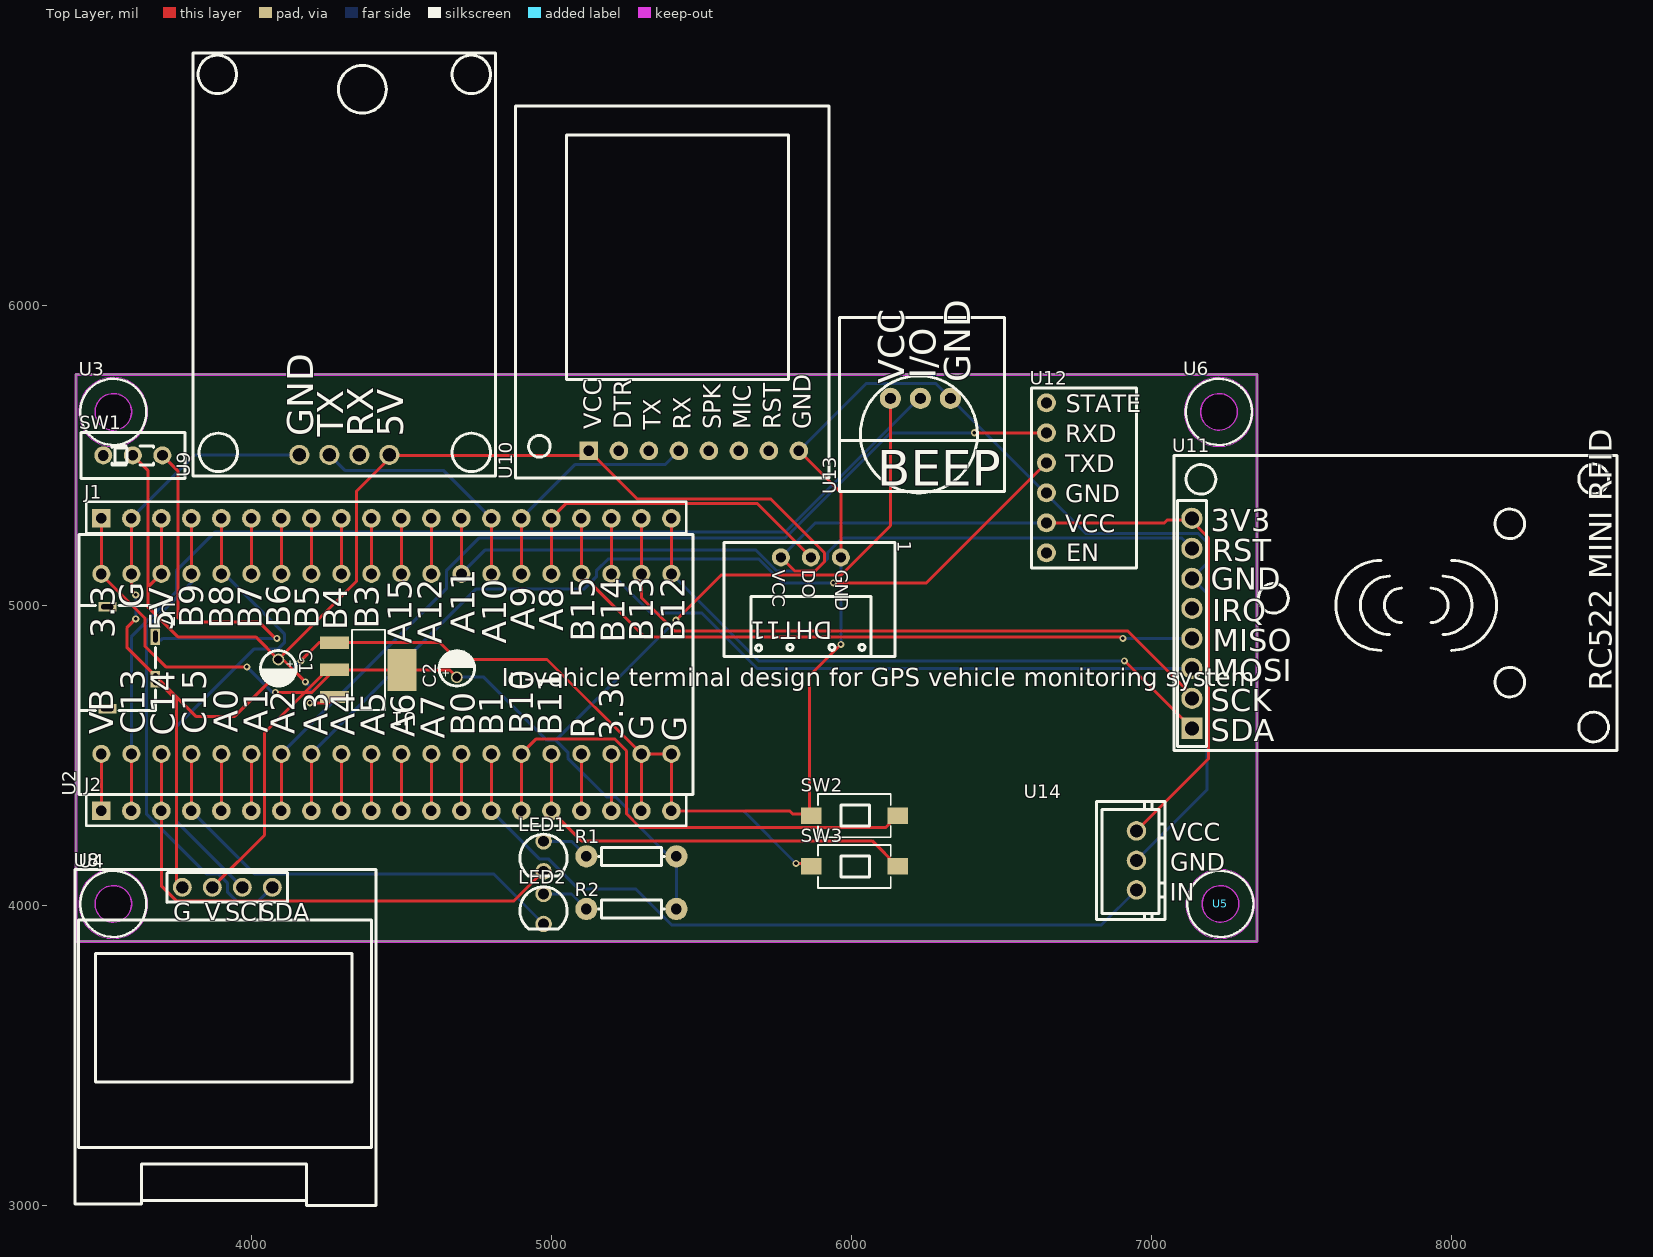
[diagram p0: Top Layer view]
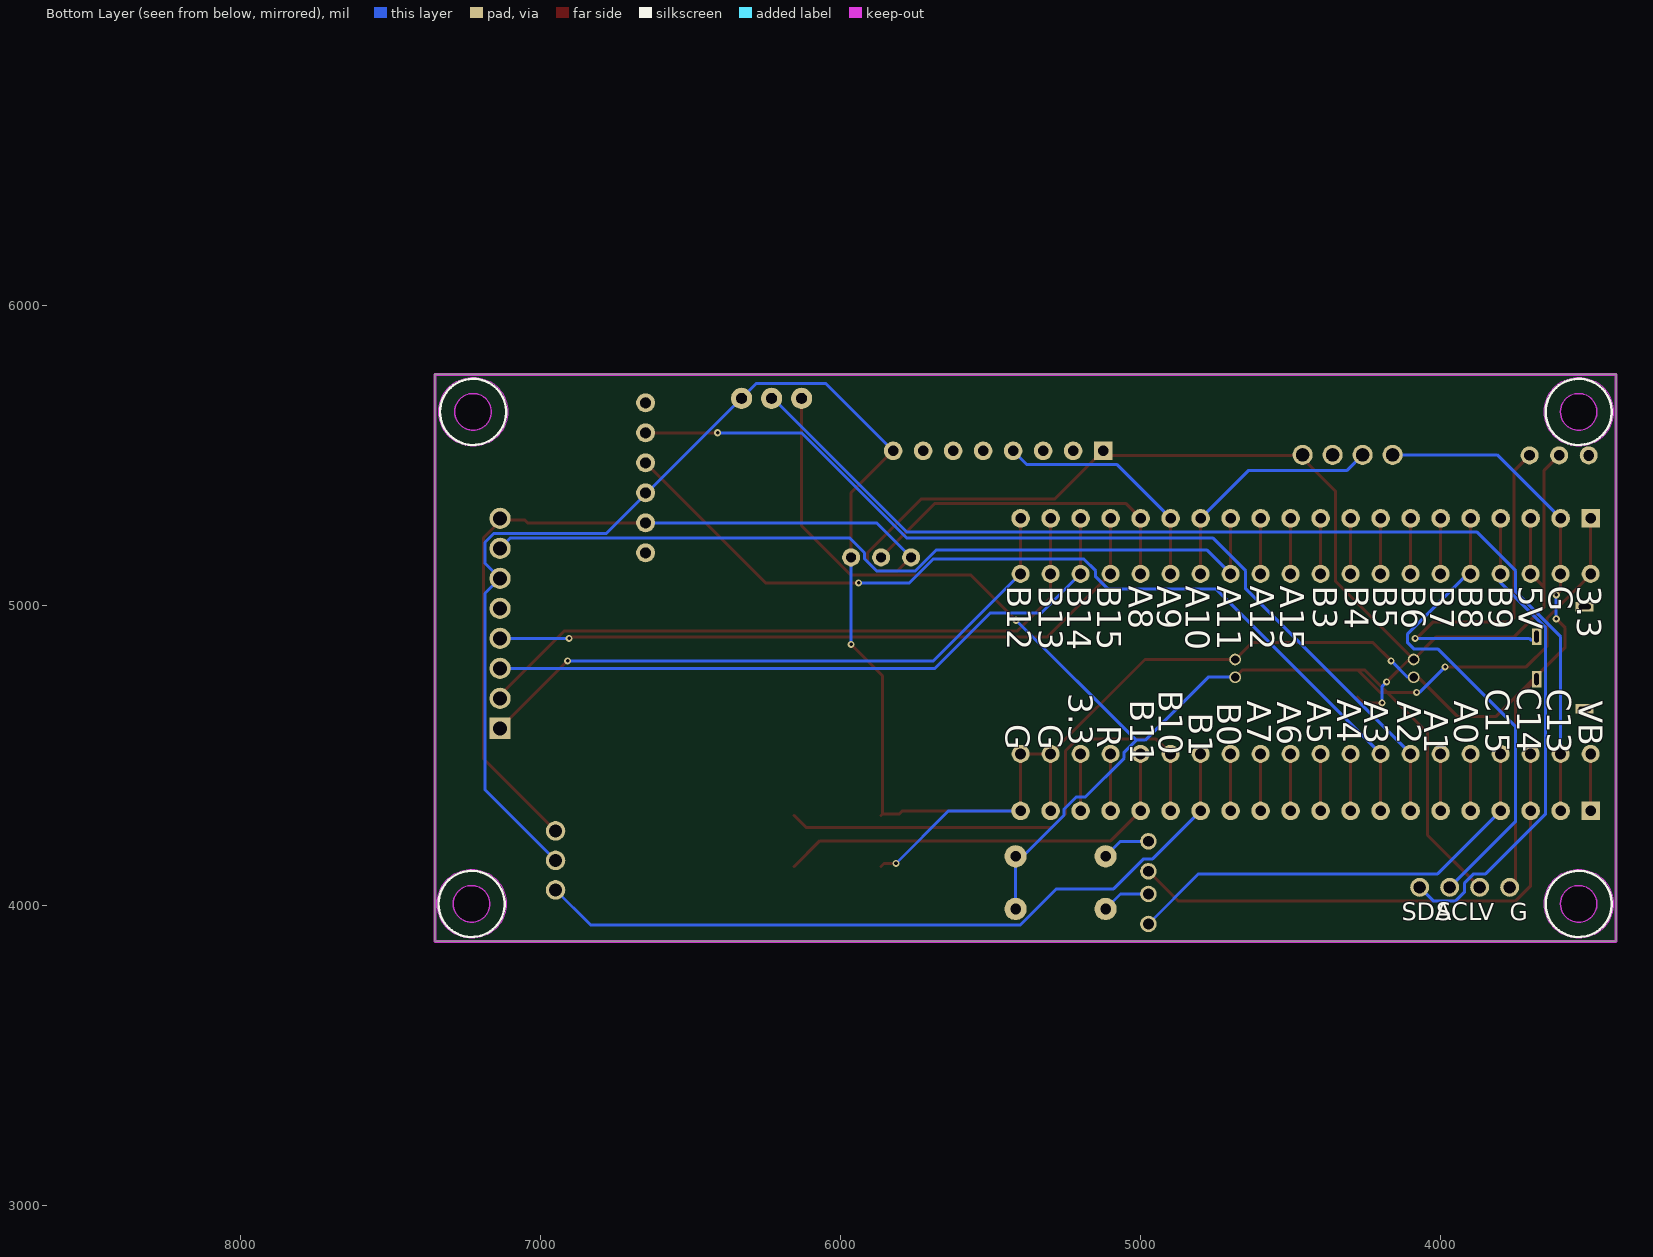
[diagram p1: Bottom Layer view, seen from below]
# Altium PCB MISC49937.pcbdoc
Units mil, origin at the board's own origin, x right, y up, seen from the top; angles counter-clockwise.
Board outline 3937.01 x 1889.76 mil, 2 copper layers (Top Layer, Bottom Layer), stack 62.206 mil thick; 26 components, 41 nets, 146 pads, 16 vias.

## Layer stack, top to bottom
Top Solder Mask Layer: solder mask 0.394, Dk 3.3
Top Layer: signal copper 1.379
Dielectric1: surface 59.449, FR4, Dk 4.5
Bottom Layer: signal copper 1.378
Bottom Solder Mask Layer: solder mask 0.394, Dk 3.3

## Board outline
3413.74,5770 3413.74,3880.24 7350.75,3880.24 7350.75,5770

## Design rules (kind name [scope] priority, off if disabled: settings)
BoardOutlineClearance copperThickness2oz_1 [All] p2 off: genericclearance=7.99 ignorepadtopadclearanceinfootprint=FALSE except(0: Arc-SplitContinuation Track-SplitContinuation SMDPad-SplitContinuation THPad-SplitContinuation Via-SplitContinuation Fill-SplitContinuation Region-SplitContinuation Poly-SplitContinuation Text-SplitContinuation Hole-SplitContinuation; 5.98: Arc-CutoutEdge SMDPad-CutoutEdge THPad-CutoutEdge Via-CutoutEdge Fill-CutoutEdge Region-CutoutEdge Text-CutoutEdge; 6.93: Hole-OutlineEdge Hole-CutoutEdge; 10: Poly-OutlineEdge Poly-CutoutEdge; 11.81: Arc-OutlineEdge Track-OutlineEdge SMDPad-OutlineEdge THPad-OutlineEdge Via-OutlineEdge Fill-OutlineEdge Region-OutlineEdge Text-OutlineEdge Track-CutoutEdge)
BoardOutlineClearance copperThickness1oz_1 [All] p4: genericclearance=4.02 ignorepadtopadclearanceinfootprint=FALSE except(0: Arc-SplitContinuation Track-SplitContinuation SMDPad-SplitContinuation THPad-SplitContinuation Via-SplitContinuation Fill-SplitContinuation Region-SplitContinuation Poly-SplitContinuation Text-SplitContinuation Hole-SplitContinuation; 6: SMDPad-CutoutEdge THPad-CutoutEdge Via-CutoutEdge Fill-CutoutEdge Region-CutoutEdge Text-CutoutEdge; 6.93: Hole-OutlineEdge Hole-CutoutEdge; 10: Poly-OutlineEdge Poly-CutoutEdge; 11.8: Arc-OutlineEdge Track-OutlineEdge SMDPad-OutlineEdge THPad-OutlineEdge Via-OutlineEdge Fill-OutlineEdge Region-OutlineEdge Text-OutlineEdge; 11.81: Arc-CutoutEdge Track-CutoutEdge)
Clearance copperThickness2oz [All] p1 off: gap=7.99 ignorepadtopadclearanceinfootprint=FALSE except(5.98: SMDPad-Track SMDPad-SMDPad THPad-Track SMDPad-THPad THPad-THPad Track-Via SMDPad-Via THPad-Via Via-Via Fill-Track Region-Track Fill-SMDPad Region-SMDPad Fill-THPad Region-THPad Fill-Via Region-Via Fill-Fill Fill-Region Region-Region Arc-Track Arc-SMDPad Arc-THPad Arc-Via Fill-Arc Region-Arc Arc-Arc Text-Track SMDPad-Text Text-THPad Text-Via Fill-Text Region-Text Arc-Text Text-Text; 6.93: Hole-Track Hole-SMDPad Hole-THPad Hole-Via Fill-Hole Region-Hole Hole-Arc Hole-Text; 10: Poly-Track Poly-SMDPad Poly-THPad Poly-Via Poly-Fill Poly-Region Poly-Poly Poly-Arc Poly-Text Poly-Hole)
Clearance copperThickness1oz [All] p3: gap=4.02 ignorepadtopadclearanceinfootprint=FALSE except(5.98: SMDPad-Track SMDPad-SMDPad THPad-Track SMDPad-THPad THPad-THPad Track-Via SMDPad-Via THPad-Via Via-Via Fill-Track Region-Track Fill-SMDPad Region-SMDPad Fill-THPad Region-THPad Fill-Via Region-Via Fill-Fill Fill-Region Region-Region; 6: Arc-Track Arc-SMDPad Arc-THPad Arc-Via Fill-Arc Region-Arc Arc-Arc Text-Track SMDPad-Text Text-THPad Text-Via Fill-Text Region-Text Arc-Text Text-Text; 6.93: Hole-Track Hole-SMDPad Hole-THPad Hole-Via Fill-Hole Region-Hole Hole-Arc Hole-Text; 10: Poly-Track Poly-SMDPad Poly-THPad Poly-Via Poly-Fill Poly-Region Poly-Poly Poly-Arc Poly-Text Poly-Hole)
DiffPairsRouting differentialPair [All] p1: maxlimit=6 minlimit=6 mostfreqgap=6 toplayer_minwidth=5 toplayer_prefwidth=10 toplayer_maxwidth=100 toplayer_mingap=6 toplayer_prefgap=6 toplayer_maxgap=6 bottomlayer_minwidth=5 bottomlayer_prefwidth=10 bottomlayer_maxwidth=100 bottomlayer_mingap=6 bottomlayer_prefgap=6 bottomlayer_maxgap=6 maxuncoupledlength=10
HoleToHoleClearance otherClearance [All] p1: gap=11.81 allowstackedmicrovias=TRUE
Length netLength [All] p1: minlimit=0 maxlimit=0
MatchedLengths netLengthTolerance [All] p1: tolerance=1000
PasteMaskExpansion pasteMaskExpansion [All] p1: expansion=0
PlaneConnect innerPlane [All] p1: planeconnectstyle=Relief reliefexpansion=20 reliefentries=4 reliefconductorwidth=10 reliefairgap=10
PolygonConnect copperRegion [All] p1: connectstyle=Relief reliefconductorwidth=10 reliefentries=4 polygonreliefangle="90 Angle" airgapwidth=10 via.connectstyle=Relief via.reliefconductorwidth=10 via.reliefentries=4 via.polygonreliefangle="90 Angle" via.airgapwidth=10
RoutingVias viaSize [All] p1: holewidth=12.01 width=24.02 viastyle="Through Hole" minholewidth=11.81 minwidth=19.68 maxholewidth=248.03 maxwidth=393.7
SolderMaskExpansion solderMaskExpansion [IsVia] p1: expansion=-1000 istentingtop=TRUE
SolderMaskExpansion solderMaskExpansion [All] p2: expansion=2 istentingtop=FALSE
Width copperThickness2oz_2 [All] p1 off: maxlimit=100 minlimit=8 preferedwidth=10
Width copperThickness1oz_2 [All] p2: maxlimit=100 minlimit=5 preferedwidth=10

## Components (designator, comment, footprint, x,y, rotation, side; value= is the part's Value field where it differs from the comment)
1 "FYS#DHT11 COPY" "FYS#DHT11_X COPY" 5893.74,5160 r270 top
C1 "1u" CAP-D3.0×F1.5 4088.74,4790 r270 top
C2 "1u" CAP-D3.0×F1.5 4683.74,4790 r90 top
J1 "HDR-M-2.54_1x20" HDR-M-2.54_1X20 4448.74,5290 r0 top
J2 "HDR-M-2.54_1x20" HDR-M-2.54_1X20 4448.74,4315 r0 top
LED1 "LED-TH-3mm_R" LED-TH_BD3.0_RED 4972.69,4163.7 r0 top
LED2 "LED-TH-3mm_R" LED-TH_BD3.0_RED 4972.69,3988.01 r0 top
R1 "1k" R_AXIAL-0.3 5265.5,4163.7 r0 top
R2 "1k" R_AXIAL-0.3 5265.5,3988.01 r0 top
SW1 "SS12D00G3" SW-TH_SS-12D01-GX 3603.74,5500 r0 top
SW2 "1TS002B-2300-5001" SW-SMD_L6.0-W3.5-LS8.0 6008.92,4299.28 r0 top
SW3 "1TS002B-2300-5001" SW-SMD_L6.0-W3.5-LS8.0 6008.92,4129.8 r0 top
U1 "AMS1117-3.3" SOT-223_L6.5-W3.5-P2.30-LS7.0-BR 4388.74,4785 r180 top
U2 "" FYS_STM32F103C最小系统 3418.74,4370 r90 top
U3 "Standoff" M3铜柱 3538.74,5645 r0 top
U4 "Standoff" M3铜柱 3538.74,4005 r0 top
U5 "Standoff" M3铜柱 7228.74,4005 r0 top
U6 "Standoff" M3铜柱 7223.74,5645 r0 top
U7 "TYPE-C 2P 90 2J 108" usb-a-th_type-c-2p-90-2j-108 3598.74,4825 r270 top
U8 "FYS#0.96 OLED IIC_4PIN COPY COPY COPY" FYS_OLED_IIC 3948.74,4060 r0 top
U9 "FYS#GPS-6M_no mounting hole" FYS#GPS模块_不带槽 4308.74,6130 r90 top
U10 "FYS#SIM900AMINI" FYS#SIM900AMINI 5538.74,5475 r90 top
U11 "FYS#RC522 MINI RFID module COPY COPY" "FYS#RC522 MINI RFID模块 COPY_1" 7073.74,5500 r0 top
U12 "FYS#HC series Bluetooth module COPY" "FYS#HC-05蓝牙模块 COPY" 6648.74,5425 r0 top
U13 "FYS#BEEP buzzer module COPY" "FYS#BEEP蜂鸣器模块 COPY" 6228.74,5530 r90 top
U14 "FYS#1-channel 5V optocoupler isolated relay module COPY" "FYS#1路5V光偶隔离继电器模块 COPY" 6948.74,4150 r0 top

## Footprints (in the part's own frame and the unit in brackets; to place one, negate y for a bottom-side part, rotate by r counter-clockwise, add the part's x,y. Pads: shape width x height; smd on the part's side, far side on the other; paste and mask are expansions set on the pad)
CAP-D3.0×F1.5 [mm]
  round 1 hole 0.7 paste+0 mask+0.102: 1(-0.751,0) 2(0.751,0)
  silkscreen extent -1.5,-1.5 1.5,1.5
"FYS#1路5V光偶隔离继电器模块 COPY" [mm]
  round 1.65 hole 1.1 paste+0 mask+0.05: 1(0,2.5) 2(0,0) 3(0,-2.5)
  silkscreen extent -3.4,-5 2.4,5
"FYS#BEEP蜂鸣器模块 COPY" [mm]
  round 1.8 hole 0.9 slot 0.9 at 90 deg: 1(4.064,2.54) 2(4.064,0) 3(4.064,-2.54)
  silkscreen extent -3.93,-7.11 10.92,6.86
"FYS#DHT11_X COPY" [mil]
  round 60 hole 31.89 slot 32.09 at 0 deg: 1(0,70) 2(0,-30) 3(0,-130)
  silkscreen extent -50,-320 330,250
FYS#GPS模块_不带槽 [mm]
  round 1.7 hole 1.1 slot 1.105 at 0 deg: 1(-15.962,3.807) 2(-15.962,1.267) 3(-15.962,-1.273) 4(-15.962,-3.813)
  silkscreen extent -17.75,-12.8 18.05,12.8
"FYS#HC-05蓝牙模块 COPY" [mm]
  round 1.6 hole 0.9 slot 0.905 at 90 deg: 1(0,6.35) 2(0,3.81) 3(0,1.27) 4(0,-1.27) 5(0,-3.81) 6(0,-6.35)
  silkscreen extent -1.27,-7.62 7.62,7.62
"FYS#RC522 MINI RFID模块 COPY_1" [mm]
  rect 1.8x1.8 hole 1.2 paste+0 mask+0.102: 1(1.524,-23.114)
  round 1.8 hole 1.2 paste+0 mask+0.102: 2(1.524,-20.574) 3(1.524,-18.034) 4(1.524,-15.494) 5(1.524,-12.954) 6(1.524,-10.414) 7(1.524,-7.874) 8(1.524,-5.334)
  silkscreen extent 0,-25 37.5,0
FYS#SIM900AMINI [mil]
  rect 62x62 hole 35 paste+0 mask+4: 1(40,415)
  round 62 hole 35 paste+0 mask+4: 2(40,315) 3(40,215) 4(40,115) 5(40,15) 6(40,-85) 7(40,-185) 8(40,-285)
  silkscreen extent -50,-385 1190,660
FYS_OLED_IIC [mm]
  round 1.6 hole 1 slot 1.005 at 0 deg: 1(-4.572,0) 2(-2.032,0) 3(0.508,0) 4(3.048,0)
  silkscreen extent -13.65,-26.92 11.81,1.5
FYS_STM32F103C最小系统 [mil]
  round 60 hole 36 paste+0 mask+4: 1(135,-80) 2(135,-180) 3(135,-280) 4(135,-380) 5(135,-480) 6(135,-580) 7(135,-680) 8(135,-780) 9(135,-880) 10(135,-980) 11(135,-1080) 12(135,-1180) 13(135,-1280) 14(135,-1380) 15(135,-1480) 16(135,-1580) 17(135,-1680) 18(135,-1780) 19(135,-1880) 20(135,-1980) 21(735,-80) 22(735,-180) 23(735,-280) 24(735,-380) 25(735,-480) 26(735,-580) 27(735,-680) 28(735,-780) 29(735,-880) 30(735,-980) 31(735,-1080) 32(735,-1180) 33(735,-1280) 34(735,-1380) 35(735,-1480) 36(735,-1580) 37(735,-1680) 38(735,-1780) 39(735,-1880) 40(735,-1980)
  silkscreen extent 0,-2052 866,-5
HDR-M-2.54_1X20 [mil]
  rect 62x62 hole 35: 1(-950,0)
  round 62 hole 35: 2(-850,0) 3(-750,0) 4(-650,0) 5(-550,0) 6(-450,0) 7(-350,0) 8(-250,0) 9(-150,0) 10(-50,0) 11(50,0) 12(150,0) 13(250,0) 14(350,0) 15(450,0) 16(550,0) 17(650,0) 18(750,0) 19(850,0) 20(950,0)
  silkscreen extent -1000,-50 1000,55
LED-TH_BD3.0_RED [mm]
  round 1.4 hole 0.9: 1(0,1.27) 2(0,-1.27)
  silkscreen extent -2,-1.69 2,1.87
M3铜柱 [mil]
  Top Layer keep-out region: -0.35,-115.47 9.15,-115.07 18.59,-113.89 27.89,-111.93 37,-109.2 45.86,-105.74 54.39,-101.56 62.56,-96.68 70.29,-91.15 77.54,-85 84.26,-78.27 90.4,-71.02 95.92,-63.27 100.78,-55.1 104.96,-46.56 108.41,-37.7 111.11,-28.58 113.06,-19.28 114.23,-9.84 114.62,-0.34 114.22,9.16 113.04,18.59 111.09,27.9 108.37,37.01 104.91,45.87 100.73,54.41 95.86,62.58 90.34,70.31 84.19,77.57 77.46,84.29 70.21,90.43 62.47,95.95 54.3,100.82 45.76,105 36.9,108.45 27.78,111.16 18.48,113.11 9.04,114.29 -0.46,114.68 -9.96,114.29 -19.39,113.11 -28.7,111.16 -37.81,108.45 -46.67,105 -55.21,100.82 -63.38,95.95 -71.12,90.43 -78.38,84.29 -85.1,77.57 -91.25,70.31 -96.78,62.58 -101.65,54.41 -105.83,45.87 -109.28,37.01 -112,27.9 -113.96,18.59 -115.14,9.16 -115.53,-0.34 -115.15,-9.84 -113.97,-19.28 -112.03,-28.58 -109.32,-37.7 -105.87,-46.56 -101.7,-55.1 -96.84,-63.27 -91.32,-71.02 -85.18,-78.27 -78.46,-85 -71.21,-91.15 -63.47,-96.68 -55.31,-101.56 -46.77,-105.74 -37.92,-109.2 -28.8,-111.93 -19.5,-113.89 -10.07,-115.07 -0.57,-115.47 -0.45,-115.47 -0.35,-115.47
  Bottom Layer keep-out region: -0.34,-114.68 9.15,-114.28 18.59,-113.1 27.89,-111.14 37,-108.42 45.86,-104.95 54.4,-100.77 62.56,-95.9 70.3,-90.36 77.55,-84.21 84.26,-77.49 90.4,-70.23 95.92,-62.48 100.79,-54.31 104.96,-45.77 108.41,-36.91 111.12,-27.79 113.06,-18.49 114.23,-9.05 114.62,0.45 114.22,9.95 113.04,19.38 111.09,28.69 108.37,37.8 104.91,46.66 100.73,55.2 95.86,63.36 90.34,71.1 84.19,78.35 77.46,85.08 70.21,91.22 62.47,96.74 54.3,101.61 45.76,105.78 36.9,109.24 27.79,111.95 18.48,113.9 9.04,115.08 -0.46,115.47 -9.96,115.08 -19.39,113.9 -28.7,111.95 -37.81,109.24 -46.67,105.78 -55.21,101.61 -63.38,96.74 -71.12,91.22 -78.38,85.08 -85.1,78.35 -91.25,71.1 -96.78,63.36 -101.64,55.2 -105.82,46.66 -109.28,37.8 -112,28.69 -113.95,19.38 -115.14,9.95 -115.53,0.45 -115.14,-9.05 -113.97,-18.49 -112.03,-27.79 -109.32,-36.91 -105.87,-45.77 -101.7,-54.31 -96.84,-62.48 -91.32,-70.23 -85.18,-77.49 -78.46,-84.21 -71.21,-90.36 -63.47,-95.9 -55.31,-100.77 -46.77,-104.95 -37.91,-108.42 -28.8,-111.14 -19.5,-113.1 -10.07,-114.28 -0.57,-114.68 -0.45,-114.68 -0.34,-114.68
  Board Outline Layer circle w0.1: c0,-0.01 r61.02
  Board Outline Layer region: 61.02,-0.01 54.98,-26.49 38.05,-47.72 13.58,-59.5 -13.58,-59.5 -38.05,-47.72 -54.98,-26.49 -61.02,-0.01 -61.02,-0.01 -54.98,26.47 -38.05,47.7 -13.58,59.48 13.58,59.48 38.05,47.7 54.98,26.47 61.02,-0.01
  Board Outline Layer region: 61.02,-0.01 60.64,-6.84 59.49,-13.59 57.6,-20.16 54.98,-26.49 51.67,-32.48 47.71,-38.06 43.15,-43.16 38.05,-47.72 32.47,-51.68 26.48,-54.99 20.15,-57.61 13.58,-59.5 6.83,-60.65 0,-61.03 -6.83,-60.65 -13.58,-59.5 -20.15,-57.61 -26.48,-54.99 -32.47,-51.68 -38.05,-47.72 -43.15,-43.16 -47.71,-38.06 -51.67,-32.48 -54.98,-26.49 -57.6,-20.16 -59.49,-13.59 -60.64,-6.84 -61.02,-0.01 -60.64,6.82 -59.49,13.57 -57.6,20.14 -54.98,26.47 -51.67,32.46 -47.71,38.04 -43.15,43.14 -38.05,47.7 -32.47,51.66 -26.48,54.97 -20.15,57.59 -13.58,59.48 -6.83,60.63 0,61.01 6.83,60.63 13.58,59.48 20.15,57.59 26.48,54.97 32.47,51.66 38.05,47.7 43.15,43.14 47.71,38.04 51.67,32.46 54.98,26.47 57.6,20.14 59.49,13.57 60.64,6.82
  Multi-Layer board cut-out: 61.02,-0.01 54.98,-26.49 38.05,-47.72 13.58,-59.5 -13.58,-59.5 -38.05,-47.72 -54.98,-26.49 -61.02,-0.01 -61.02,-0.01 -54.98,26.47 -38.05,47.7 -13.58,59.48 13.58,59.48 38.05,47.7 54.98,26.47 61.02,-0.01
  silkscreen extent -110,-110 110,110
R_AXIAL-0.3 [mil]
  round 74 hole 35.4: 1(-150,0) 2(150,0)
  silkscreen extent -110,-30 110,30
SOT-223_L6.5-W3.5-P2.30-LS7.0-BR [mm]
  rect 2.465x1.05 smd: 1(2.858,-2.3) 2(2.857,0) 3(2.857,2.3)
  rect 2.465x3.54 smd: 4(-2.857,0)
  silkscreen extent -1.4,-3.4 1.4,3.4
SW-SMD_L6.0-W3.5-LS8.0 [mm]
  rect 1.74x1.4 smd: 1(-3.67,0) 2(3.67,0)
  silkscreen extent -3.08,-1.83 3.08,1.83
SW-TH_SS-12D01-GX [mil]
  round 60 hole 36: 1(-98.42,-0.01) 2(-0.01,0.01) 3(98.42,0)
  silkscreen extent -173,-77 173,77
usb-a-th_type-c-2p-90-2j-108 [mm]
  rect 1.4x0.8 hole 0.36 slot 1 at 0 deg: 2(1.8,2.04) 3(-1.8,2.04)
  rect 0.8x1.524 hole 0.4 slot 1.05 at 90 deg: 4(4.325,-2.04) 5(-4.325,-2.04)
  silkscreen extent -4.45,-4.44 4.44,2.04

## Via types
v1: diameter 24.02, hole 12, Top Layer to Bottom Layer, 16 vias

## Nets (pads, with @x,y where several pads share a name; then routed paths per layer and width w, separated by ;. In a path a pad name is that pad's centre, name@x,y a point inside that pad or via, vN(x,y) a via of type N, cw(c..) or ccw(c..) an arc to the next point about the centre after c; other vN are vias at no path point)
$1N2: SW1.3 U7.3 | length 1327.3
  Top Layer w10: SW1.3 3753.74,5448.42 3753.74,4960 3768.74,4945 4023.74,4945 v1@4078.74,4890
  Bottom Layer w10: U7.3 3679.06,4894.69 3688.74,4885 3698.74,4885 3703.74,4890 v1(4083.74,4890)
$1N26: J2.1 U2.1 | length 190
  Top Layer w10: J2.1 U2.1
$1N42: J2.17 U2.17 | length 190
  Top Layer w10: J2.17 U2.17
$1N43: J2.18 U2.18 | length 190
  Top Layer w10: J2.18 U2.18
$1N70: LED2.1 R2.1 | length 163.5
  Bottom Layer w10: LED2.1 5065.5,4038.01 R2.1
$1N73: LED1.1 R1.1 | length 163.5
  Bottom Layer w10: LED1.1 5065.5,4213.7 R1.1
+3.3V: C2.1 J1.1 R1.2 R2.2 U1.2 U1.4 U2.21 U8.2 U13.1 | length 5554.5
  Top Layer w10: U2.21@3498.74,5100 U2.21@3498.74,5102.52 ; J1.1 U2.21 U2.21@3498.74,5102.52 ; U8.2 4042.72,4233.98 4042.72,4575 4177.72,4710 ; v1(3983.74,4795) 3713.57,4795 3643.74,4864.82 3643.74,4957.52 U2.21@3498.74,5102.52 ; v1(4078.74,4710) 4177.72,4710 ; C2.1 4659.19,4785 U1.4 U1.2 ; v1(5413.74,4950.45) 5563.74,5100.45 5963.74,5100.45 6128.74,5265.45 U13.1 ; 4177.72,4710 4201.24,4710 U1.2 ; 4177.72,4710 4252.72,4785 U1.2
  Bottom Layer w10: v1(3983.74,4795) 4068.74,4710 v1(4078.74,4710) ; C2.1@4683.75,4760.45 4773.75,4760.45 4983.74,4550.45 5013.74,4550.45 ; v1(5413.74,4950.45) 5013.74,4550.45 ; R2.2 R1.2 5390.5,4163.7 5253.74,4300.45 5253.74,4320.45 5213.74,4360.45 5183.74,4360.45 5053.74,4490.45 5053.74,4510.45 5013.74,4550.45
+5V: 1.3 C1.1 J1.3 SW1.2 U1.3 U2.23 U9.4 U10.1 U11.8 U12.5 U14.1 | length 6800.8
  Top Layer w10: SW1.2 3653.74,5449.99 3653.74,5060 ; U2.23@3698.74,5100 U2.23 ; J1.3 U2.23 ; v1(4178.74,4745) 4104.19,4819.55 C1.1 ; v1(4193.74,4675) 4256.79,4675 U1.3 ; U9.4 4460.88,5499.55 U9.4@4468.74,5499.55 ; 1.3 5808.74,5115 5878.74,5115 5908.74,5145 5908.74,5175 5728.74,5355 5283.74,5355 U10.1 5108.3,5499.55 U9.4@4468.74,5499.55 ; U12.5 7042.45,5275 7052.45,5285 U11.8@7128.74,5285 ; U14.1 7188.74,4488.43 7188.74,5225 U11.8@7128.74,5285 ; U11.8 U11.8@7128.74,5285 ; 3653.74,5060 3653.74,4995 3753.74,4895 4013.29,4895 C1.1 ; 3653.74,5060 U2.23 ; C1.1 4348.74,5079.55 4348.74,5379.55 U9.4@4468.74,5499.55
  Bottom Layer w10: v1(4178.74,4745) 4193.74,4730 v1(4193.74,4675) ; 1.3 5878.74,5275 U12.5
GND: 1.1 C1.2 C2.2 J1.2 J2.19 J2.20 SW2.1 SW3.1 U1.1 U2.19 U2.20 U2.22 U7.2 U8.1 U9.1 U10.8 U11.6 U12.4 U13.3 U14.2 | length 9575.7
  Top Layer w10: J1.2 U2.22 3598.74,5050 v1(3613.74,5035) ; v1(3613.74,4955) 3583.74,4925 3583.74,4860 3813.74,4630 3943.29,4630 4073.74,4760.45 v1(4088.74,4760.45) ; U7.2 3748.74,4684.45 3748.74,4080 U8.1 ; v1(4163.74,4815) 4224.29,4875.55 U1.1 4627.74,4875.55 C2.2 4984.19,4819.55 U2.19 ; J2.19 U2.19 ; v1(5813.94,4139.8) 5854.43,4139.8 SW3.1 ; U10.8 5963.74,5375 1.1 ; SW2.1 SW2.1@5858.74,4305 ; v1(5963.74,4870) 5858.74,4765 SW2.1@5858.74,4305 ; U2.19 U2.20 J2.20 5792.44,4315 5802.44,4305 SW2.1@5858.74,4305
  Bottom Layer w10: J1.2 3810.31,5501.57 U9.1 ; v1(3613.74,4955) v1(3613.74,5035) ; v1(4088.74,4760.45) 4109.19,4760.45 v1(4163.74,4815) ; J2.20 5638.74,4315 v1(5813.94,4139.8) ; U10.8 6048.74,5740 6278.74,5740 U13.3 U12.4@6643.74,5375 ; v1(5963.74,4870) 1.1 ; U12.4 U12.4@6643.74,5375 ; U14.2 7183.74,4385 7183.74,5040 U11.6 7183.74,5140 7183.74,5210.01 7153.74,5240.01 6778.74,5240.01 U12.4@6643.74,5375
PA0: J2.5 U2.5 | length 190
  Top Layer w10: J2.5 U2.5
PA1: J2.6 U2.6 | length 190
  Top Layer w10: J2.6 U2.6
PA2: J2.7 U2.7 U12.2 | length 3218.4
  Top Layer w10: J2.7 U2.7 ; v1(6408.74,5575) U12.2
  Bottom Layer w10: U2.7 4648.74,5055 4648.74,5115 4758.74,5225 5778.74,5225 6128.74,5575 v1(6408.74,5575)
PA3: J2.8 U2.8 U12.3 | length 3119.8
  Top Layer w10: J2.8 U2.8 ; v1(5938.74,5075) 6248.74,5075 U12.3
  Bottom Layer w10: U2.8 4748.74,5055 5108.74,5055 5148.74,5095 5148.74,5115 5188.74,5155 5688.74,5155 5768.74,5075 v1(5938.74,5075)
PA4: J2.9 U2.9 | length 190
  Top Layer w10: J2.9 U2.9
PA5: J2.10 U2.10 | length 190
  Top Layer w10: J2.10 U2.10
PA6: J2.11 U2.11 | length 190
  Top Layer w10: J2.11 U2.11
PA7: J2.12 U2.12 | length 190
  Top Layer w10: J2.12 U2.12
PA8: 1.2 J1.16 U2.36 | length 1150.3
  Top Layer w10: U2.36@4998.74,5100 J1.16 5048.74,5340 5683.74,5340 1.2
PA9: J1.15 U2.35 U10.4 | length 808.2
  Top Layer w10: U2.35@4898.74,5100 J1.15
  Bottom Layer w10: J1.15 5078.74,5470 5378.74,5470 U10.4
PA10: J1.14 U2.34 U9.2 | length 817.5
  Top Layer w10: U2.34@4798.74,5100 J1.14
  Bottom Layer w10: U9.2 4310.43,5450 4638.75,5450 J1.14
PA11: J1.13 U2.33 U11.7 | length 2758.9
  Top Layer w10: U2.33@4698.74,5100 J1.13
  Bottom Layer w10: U2.33 4778.75,5185 5678.74,5185 5748.74,5115 5878.74,5115 5918.74,5155 5918.74,5175 5968.74,5225 7098.69,5225 U11.7
PA12: J1.12 U2.32 | length 190
  Top Layer w10: U2.32@4598.74,5100 J1.12
PA15: J1.11 U2.31 | length 190
  Top Layer w10: U2.31@4498.74,5100 J1.11
PB0: J2.13 U2.13 | length 190
  Top Layer w10: J2.13 U2.13
PB1: J2.14 U2.14 U14.3 | length 2545.7
  Top Layer w10: J2.14 U2.14
  Bottom Layer w10: J2.14 4958.74,4155 4988.74,4155 5088.74,4055 5278.74,4055 5398.74,3935 6832.17,3935 U14.3@6948.74,4051.57
PB3: J1.10 U2.30 | length 190
  Top Layer w10: U2.30@4398.74,5100 J1.10
PB4: J1.9 U2.29 | length 190
  Top Layer w10: U2.29@4298.74,5100 J1.9
PB5: J1.8 U2.28 | length 190
  Top Layer w10: U2.28@4198.74,5100 J1.8
PB6: J1.7 U2.27 | length 190
  Top Layer w10: U2.27@4098.74,5100 J1.7
PB7: J1.6 U2.26 | length 190
  Top Layer w10: U2.26@3998.74,5100 J1.6
PB8: J1.5 U2.25 U8.3 | length 1614.9
  Top Layer w10: U2.25@3898.74,5100 J1.5
  Bottom Layer w10: U2.25 3908.74,5105 4108.74,4905 4108.74,4875 4088.74,4855 4008.74,4855 3748.74,4595 3748.74,4280 U8.3
PB9: J1.4 U2.24 U8.4 | length 1628.5
  Top Layer w10: U2.24@3798.74,5100 J1.4
  Bottom Layer w10: U2.24 3798.74,5075 3648.74,4925 3648.74,4305 3848.74,4105 3888.74,4105 3918.74,4075 3918.74,4045 3948.74,4015 4023.74,4015 U8.4
PB10: J2.15 SW2.2 U2.15 | length 1727.5
  Top Layer w10: J2.15 U2.15 4948.74,4555 5208.74,4555 5248.74,4515 5248.74,4305 5294.46,4259.28 6113.42,4259.28 SW2.2
PB11: J2.16 SW3.2 U2.16 | length 1421.4
  Top Layer w10: U2.16 J2.16 5098.74,4215 6068.22,4215 SW3.2
PB12: J1.20 U2.40 U11.1 | length 2138.3
  Top Layer w10: U2.40@5398.74,5100 J1.20 ; v1(6908.74,4815) U11.1
  Bottom Layer w10: U2.40 5688.74,4815 v1(6908.74,4815)
PB13: J1.19 U2.39 U11.2 | length 2249.6
  Top Layer w10: U2.39@5298.74,5100 J1.19 ; U2.39 5298.74,5025 5408.74,4915 6918.74,4915 7128.74,4705 7128.74,4695.01 U11.2
PB14: J1.18 U2.38 U11.3 | length 2255.5
  Top Layer w10: U2.38@5198.74,5100 J1.18
  Bottom Layer w10: U2.38 5328.74,4975 5498.74,4975 5683.74,4790 U11.3
PB15: J1.17 U2.37 U11.4 | length 2314.1
  Top Layer w10: U2.37@5098.74,5100 J1.17 ; U2.37 5308.74,4895 6898.74,4895 v1(6903.74,4890)
  Bottom Layer w10: v1(6903.74,4890) U11.4
PC13: J2.2 U2.2 U13.2 | length 3580.3
  Top Layer w10: J2.2@3598.74,4320 U2.2@3598.74,4510
  Bottom Layer w10: U2.2 3598.74,4895 3748.74,5045 3748.74,5115 3878.74,5245 5778.74,5245 6223.74,5690 U13.2
PC14: J2.3 LED1.2 U2.3 | length 1775.5
  Top Layer w10: U2.3 J2.3 3698.75,4065 3748.75,4015 4873.99,4015 LED1.2
PC15: J2.4 LED2.2 U2.4 | length 1520.1
  Top Layer w10: J2.4 U2.4
  Bottom Layer w10: J2.4 4008.75,4105 4805.7,4105 LED2.2
pads on no net: SW1.1 U7.4 U7.5 U9.3 U10.2 U10.3 U10.5 U10.6 U10.7 U11.5 U12.1 U12.6

## Keep-outs
Board Outline Layer:
  the board outline again, w10

## Silkscreen, mask and mechanical layers (free items; w line width, h text height)
Top Silkscreen Layer:
  text "In-vehicle terminal design for GPS vehicle monitoring system" at 4833.74,4730 h60

## Dimensions
3000,3880.24 to 3000,4825.12 on Document Layer
3278.74,5770 to 3278.74,3880.24 on Document Layer